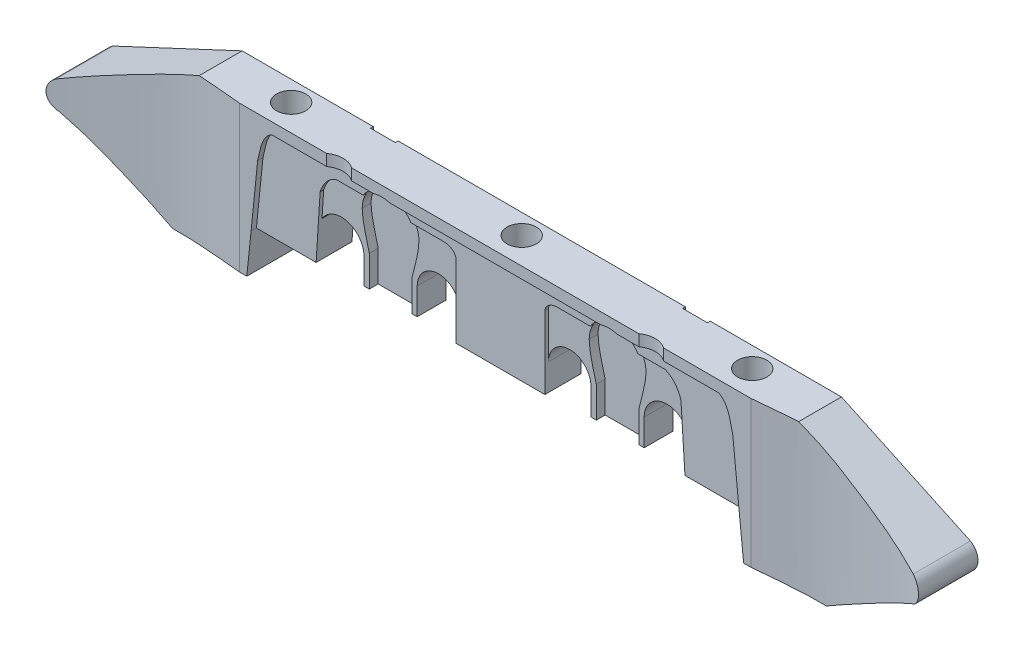
SolidWorks part; units mm, degrees
ref_plane "前视基准面" through (0, 0, 0) normal (0, 0, 1) x (1, 0, 0)
ref_plane "上视基准面" through (0, 0, 0) normal (0, 1, 0) x (1, 0, 0)
ref_plane "右视基准面" through (0, 0, 0) normal (1, 0, 0) x (0, 0, -1)
sketch "草图1" plane through (0, 0, 0) normal (0, 1, 0) x (1, 0, 0)
  line L1 (492, 0) -> (492, -52.5)
  line L6 (0, 0) -> (-1, -52.5)
  line L7 (-1, -52.5) -> (-1, -67.5)
  line L10 (492, 0) -> (330, 0)
  line L11 (330, 0) -> (330, -3.15)
  line L12 (330, -3.15) -> (302, -3.15)
  line L13 (302, -3.15) -> (302, 0)
  line L14 (302, 0) -> (0, 0)
  line L16 (330, -52.5) -> (492, -52.5)
  line L17 (203.6889, -52.5) -> (302, -52.5)
  arc A1 (302, -52.5) -> (330, -52.5) centre (316, -71.7752) cw
  spline S0 degree 3 poles (-1, -67.5) (16.2704, -61.5702) (46.0738, -55.0351) (86.8917, -50.4463) (137.4018, -45.5036) (176.0842, -50.0739) (203.6889, -52.5) knots 0 0 0 0 0.264705 0.440852 0.596046 1 1 1 1
extrude "凸台-拉伸1" add sketch "草图1" against normal blind 165
sketch3d "3D草图1"
  point P0 (492, -128.104, 30.3693)
ref_plane "基准面1" through (492, 0, 0) normal (1, 0, 0) x (0, 0, -1)
mirror "镜向2" about plane through (492, -165, 0) normal (1, 0, 0) of "凸台-拉伸1"
sketch "草图2" plane through (0, 0, 0) normal (0, 1, 0) x (1, 0, 0)
  line L0 (492, -6.13) -> (492, -39.13)
  arc A0 (492, -6.13) -> (492, -39.13) centre (492, -22.63) ccw
  circle A1 centre (232, -22.63) radius 16.5
extrude "切除-拉伸1" cut sketch "草图2" against normal blind 25
mirror "镜向3" about plane through (492, 0, 0) normal (1, 0, 0) of "切除-拉伸1"
sketch "草图3" plane through (0, 0, 0) normal (0, 1, 0) x (1, 0, 0)
  line L0 (492, -10.13) -> (492, -35.13)
  arc A0 (492, -10.13) -> (492, -35.13) centre (492, -22.63) ccw
  circle A1 centre (232, -22.63) radius 12.5
extrude "切除-拉伸2" cut sketch "草图3" against normal blind 50
sketch "草图4" plane through (0, 0, 0) normal (0, 1, 0) x (1, 0, 0)
  line L0 (492, -35.13) -> (492, -10.13) construction
  line L1 (492, -35.13) -> (492, -10.13) construction
  line L2 (492, -17.63) -> (492, -27.63)
  arc A0 (492, -17.63) -> (492, -27.63) centre (492, -22.63) ccw
  circle A1 centre (232, -22.63) radius 5
extrude "切除-拉伸3" cut sketch "草图4" against normal through all contours A1 | L2 A0
mirror "镜向4" about plane through (492, 0, 0) normal (1, 0, 0) of "切除-拉伸3", "切除-拉伸2"
sketch3d "3D草图2"
  point P0 (451.3405, -110.9349, 52.5)
ref_plane "基准面2" through (0, 0, 52.5) normal (0, 0, 1) x (1, 0, 0)
sketch3d "3D草图3"
  point P0 (521.9436, -101.4447, 0)
ref_plane "基准面3" through (0, 0, 0) normal (0, 0, -1) x (-1, 0, 0)
sketch "草图5" plane through (0, 0, 0) normal (0, 0, -1) x (-1, 0, 0)
  line L0 (-985, 0) -> (-830, 0)
  line L1 (-682, 0) -> (-984, 0) construction
  line L5 (-984, -165) -> (-984, 0) construction
  line L12 (-830, 0) -> (-975.0263, -67.8132)
  line L13 (-972.9204, -98.6514) -> (-860.6678, -165)
  line L14 (-682, -165) -> (-984, -165) construction
  line L15 (-985, -165) -> (-860.6678, -165)
  line L16 (-985, -165) -> (-985, 0)
  line L17 (-975.0263, -67.8132) -> (-975.4274, -68.0007)
  arc A0 (-984, -82.5) -> (-975.4274, -68.0007) centre (-967.0416, -82.7427) cw
  arc A1 (-984, -82.5) -> (-972.9204, -98.6514) centre (-967.0416, -82.7427) ccw
extrude "切除-拉伸4" cut sketch "草图5" against normal through all
sketch "草图7" plane through (0, 0, 52.5) normal (0, 0, 1) x (1, 0, 0)
  line L1 (330, -165) -> (654, -165) construction
  line L2 (780.3111, -165) -> (682, -165) construction
  line L7 (492, -165) -> (772.181, -165)
  line L8 (492, -15) -> (744.1036, -15)
  line L9 (759.7485, -45.6392) -> (772.181, -165)
  line L10 (492, -15) -> (492, -165)
  line L11 (492, -118.4479) -> (767.3322, -118.4479)
  spline S0 degree 2 poles (744.1036, -15) (753.7765, -19.378) (755.7084, -29.0043) knots 0 0 0 1 1 1
  spline S1 degree 2 poles (755.7084, -29.0043) (759.5639, -36.7871) (759.7485, -45.6392) knots 0 0 0 1 1 1
extrude "切除-拉伸6" cut sketch "草图7" against normal blind 26.25
sketch "草图12" plane through (0, 0, 52.5) normal (0, 0, 1) x (1, 0, 0)
  line L2 (492, -12.7591) -> (744.1036, -12.7591)
  line L4 (492, -12.7591) -> (492, -118.4479)
  line L5 (492, -118.4479) -> (767.3322, -118.4479)
  line L6 (767.3322, -118.4479) -> (759.9339, -45.9706)
  spline S0 degree 3 poles (744.1036, -12.7591) (748.9016, -15.2591) (756.5027, -26.0613) (758.1039, -38.8643) (759.9339, -45.9706) knots 0 0 0 0 0.415607 1 1 1 1
sketch3d "3D草图5"
  point P0 (585.9687, -201.3517, 26.25)
ref_plane "基准面5" through (0, 0, 26.25) normal (0, 0, 1) x (1, 0, 0)
mirror "镜向6" about plane through (0, 0, 26.25) normal (0, 0, 1) of "切除-拉伸6"
extrude "切除-拉伸17" cut sketch "草图12" against normal blind 6
sketch "草图22" plane through (0, 0, 52.5) normal (0, 0, 1) x (1, 0, 0)
  line L1 (492, -118.4479) -> (767.3322, -118.4479) construction
  line L2 (542, -118.4479) -> (700, -118.4479)
  line L3 (542, -118.4479) -> (542, -36.4479)
  line L4 (555.9068, -26.1076) -> (677.1688, -26.1076)
  line L5 (695.4822, -47.2386) -> (700, -118.4479)
  spline S0 degree 3 poles (542, -36.4479) (542.7962, -29.7542) (549.8233, -26.0722) (555.9068, -26.1076) knots 0 0 0 0 1 1 1 1
  spline S1 degree 3 poles (677.1688, -26.1076) (686.6563, -29.143) (692.7388, -38.1488) (695.4822, -47.2386) knots 0 0 0 0 1 1 1 1
extrude "切除-拉伸18" cut sketch "草图22" against normal blind 10
mirror "镜向7" about plane through (492, 0, 0) normal (1, 0, 0) of "切除-拉伸4"
mirror "镜向8" about plane through (492, 0, 0) normal (1, 0, 0) of "切除-拉伸6"
mirror "镜向9" about plane through (984, 0, 26.25) normal (0, 0, 1) of "镜向8"
mirror "镜向10" about plane through (492, 0, 0) normal (1, 0, 0) of "切除-拉伸18", "切除-拉伸17"
mirror "镜向11" about plane through (0, 0, 26.25) normal (0, 0, 1) of "镜向10", "切除-拉伸17", "切除-拉伸18"
sketch "草图23" plane through (0, 0, 52.5) normal (0, 0, 1) x (1, 0, 0)
  line L0 (442, -118.4479) -> (394, -118.4479)
  line L1 (442, -118.4479) -> (284, -118.4479) construction
  line L2 (394, -118.4479) -> (394, -88.4479)
  line L3 (442, -36.4479) -> (442, -118.4479) construction
  line L4 (442, -88.4479) -> (442, -118.4479)
  line L6 (590, -118.4479) -> (590, -88.4479)
  line L7 (542, -118.4479) -> (542, -88.4479)
  line L8 (542, -36.4479) -> (542, -118.4479) construction
  line L9 (650, -118.4479) -> (700, -118.4479)
  line L10 (542, -118.4479) -> (700, -118.4479) construction
  line L11 (700, -118.4479) -> (695.4822, -47.2386) construction
  line L12 (650, -118.4479) -> (650, -88.4479)
  line L15 (542, -118.4479) -> (590, -118.4479)
  line L16 (697.2524, -75.1407) -> (700, -118.4479)
  line L17 (334, -118.4479) -> (284, -118.4479)
  line L18 (334, -118.4479) -> (334, -88.4479)
  line L21 (284, -118.4479) -> (288.5178, -47.2386) construction
  line L23 (286.6823, -76.1688) -> (284, -118.4479)
  arc A0 (394, -88.4479) -> (442, -88.4479) centre (418, -88.4479) cw
  arc A2 (334, -88.4479) -> (286.6823, -76.1688) centre (308.5157, -89.3428) ccw
  arc A3 (542, -88.4479) -> (590, -88.4479) centre (566, -88.4479) cw
  arc A6 (650, -88.4479) -> (697.2524, -75.1407) centre (675.5, -88.4479) cw
extrude "切除-拉伸19" cut sketch "草图23" against normal through all
sketch "草图24" plane through (0, 0, 52.5) normal (0, 0, 1) x (1, 0, 0)
  line L0 (620, -118.4479) -> (644, -118.4479)
  line L1 (590, -118.4479) -> (650, -118.4479) construction
  line L2 (644, -118.4479) -> (644, -83.4479)
  line L3 (620, -118.4479) -> (596, -118.4479)
  line L4 (596, -118.4479) -> (596, -83.4479)
  arc A0 (652, -43.3957) -> (588, -43.3957) centre (620, -43.3957) ccw
  spline S0 degree 3 poles (588, -43.3957) (588.361, -57.1634) (592.8914, -70.1976) (596, -83.4479) knots 0 0 0 0 1 1 1 1
  spline S1 degree 3 poles (652, -43.3957) (651.639, -57.1634) (647.1086, -70.1976) (644, -83.4479) knots 0 0 0 0 1 1 1 1
extrude "切除-拉伸20" cut sketch "草图24" against normal blind 20
mirror "镜向12" about plane through (492, 0, 0) normal (1, 0, 0) of "切除-拉伸20"
mirror "镜向13" about plane through (0, 0, 26.25) normal (0, 0, 1) of "切除-拉伸20", "镜向12"
